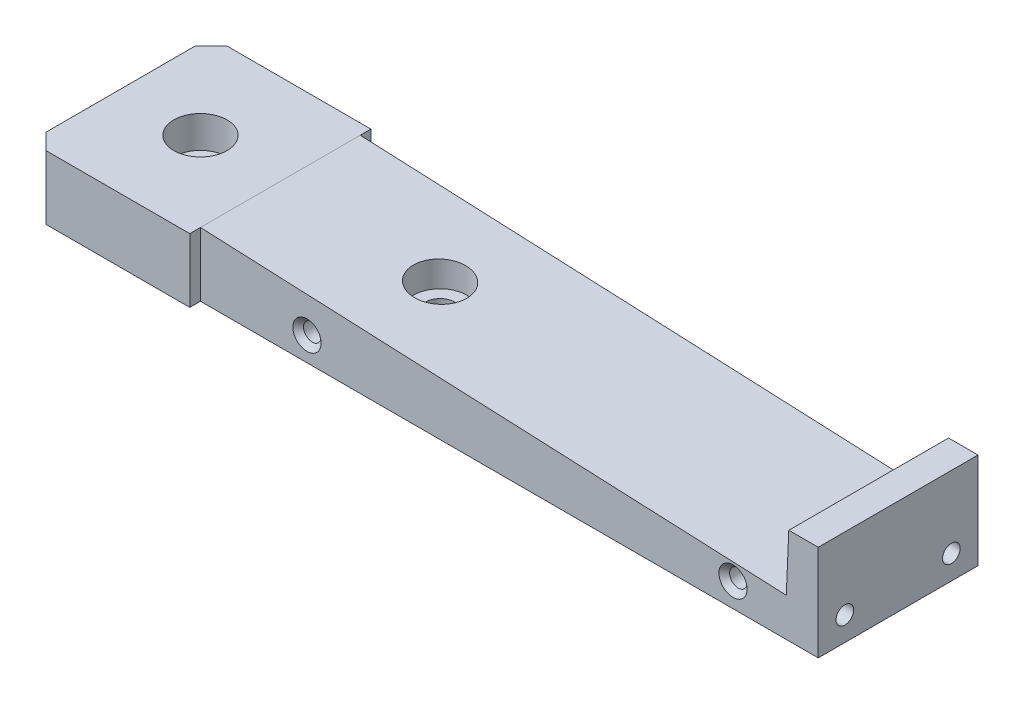
from build123d import *

# Parameters (mm, degrees)
SKETCH1_W                                            = 146
SKETCH1_H                                            = 34
BOSS_EXTRUDE1_DEPTH                                  = 6
HOLE_SIZE_PER_SOCKET_HEAD_CAP_SCREW_TYPE_D           = 5.5
HOLE_SIZE_PER_SOCKET_HEAD_CAP_SCREW_TYPE_CBORE_D     = 10
HOLE_SIZE_PER_SOCKET_HEAD_CAP_SCREW_TYPE_CBORE_DEPTH = 6
M4_TAPPED_HOLE2_D                                    = 3.3
M4_TAPPED_HOLE2_DEPTH                                = 10.1
M4_TAPPED_HOLE2_TIP                                  = 0.991420021
CHAMFER1_SIZE                                        = 3
SKETCH8_W                                            = 116
SKETCH8_H                                            = 2
CUT_EXTRUDE1_DEPTH                                   = 76.907838857
M4_TAPPED_HOLE3_AT_2_COUNT                           = 2
M4_TAPPED_HOLE3_AT_2_PITCH                           = 80
SKETCH11_W                                           = 6
SKETCH11_H                                           = 30
BOSS_EXTRUDE2_DEPTH                                  = 6
CUT_EXTRUDE2_DEPTH                                   = 82.418671077
CUT_EXTRUDE3_DEPTH                                   = 82.418671077
CHAMFER2_SIZE                                        = 1


with BuildPart() as part:
    # Sketch1 → Boss-Extrude1 (new, symmetric)
    with BuildSketch(Plane(origin=(0, 0, 0), x_dir=(1, 0, 0), z_dir=(0, 1, 0))):
        Rectangle(SKETCH1_W, SKETCH1_H)
    extrude(amount=BOSS_EXTRUDE1_DEPTH, both=True)

    # Hole size per socket head cap screw type1 (through all)
    with Locations(Plane(origin=(0, 6, 0), x_dir=(1, 0, 0), z_dir=(0, 1, 0))):
        with Locations((-58, 0), (-13, 0)):
            CounterBoreHole(HOLE_SIZE_PER_SOCKET_HEAD_CAP_SCREW_TYPE_D / 2, HOLE_SIZE_PER_SOCKET_HEAD_CAP_SCREW_TYPE_CBORE_D / 2, HOLE_SIZE_PER_SOCKET_HEAD_CAP_SCREW_TYPE_CBORE_DEPTH)

    # M4 Tapped Hole2
    with Locations(Plane(origin=(73, 0, 0), x_dir=(0, 0, -1), z_dir=(1, 0, 0))):
        with Locations((-10, -1.5), (10, -1.5)):
            Hole(M4_TAPPED_HOLE2_D / 2, depth=M4_TAPPED_HOLE2_DEPTH)
            with Locations((0, 0, -(M4_TAPPED_HOLE2_DEPTH + M4_TAPPED_HOLE2_TIP / 2))):  # 118° drill point
                Cone(0, M4_TAPPED_HOLE2_D / 2, M4_TAPPED_HOLE2_TIP, mode=Mode.SUBTRACT)

    # Chamfer1
    chamfer1_edges = [part.edges().sort_by_distance(p)[0] for p in [
        (-73, 0, 17),
        (-73, 0, -17),
    ]]
    chamfer(chamfer1_edges, length=CHAMFER1_SIZE)

    # Sketch8 → Cut-Extrude1 (cut, through all)
    with BuildSketch(Plane(origin=(0, 6, 0), x_dir=(1, 0, 0), z_dir=(0, 1, 0))):
        with Locations((15, -16)):
            Rectangle(SKETCH8_W, SKETCH8_H)
        with Locations((15, 16)):
            Rectangle(SKETCH8_W, SKETCH8_H)
    extrude(amount=-CUT_EXTRUDE1_DEPTH, mode=Mode.SUBTRACT)

    # Sketch9 → M4 Tapped Hole3 (revolve, cut)
    with BuildSketch(Plane(origin=(-23, -1.5, 15), x_dir=(0, -1, 0), z_dir=(1, 0, 0))):
        Polygon((0, 0), (0, 11.091420021), (1.65, 10.1), (1.65, 0), align=None)
    m4_tapped_hole3 = revolve(axis=Axis((-23, -1.5, 21.35), (0, 0, -1)), mode=Mode.SUBTRACT)

    # M4 Tapped Hole3 at 2: M4 Tapped Hole3 ×2
    with Locations(*[(i * M4_TAPPED_HOLE3_AT_2_PITCH, 0, 0) for i in range(1, M4_TAPPED_HOLE3_AT_2_COUNT)]):
        add(m4_tapped_hole3, mode=Mode.SUBTRACT)

    # Mirror1: M4 Tapped Hole3 across plane
    add(m4_tapped_hole3.mirror(Plane.XY), mode=Mode.SUBTRACT)

    # Mirror1 copy 1 sketch → Mirror1 copy 1 (revolve, cut)
    with BuildSketch(Plane(origin=(57, -1.5, -15), x_dir=(0, -1, 0), z_dir=(1, 0, 0))):
        Polygon((0, 0), (0, -11.091420021), (1.65, -10.1), (1.65, 0), align=None)
    revolve(axis=Axis((57, -1.5, -21.35), (0, 0, -1)), mode=Mode.SUBTRACT)

    # Sketch11 → Boss-Extrude2 (add)
    with BuildSketch(Plane(origin=(0, 6, 0), x_dir=(1, 0, 0), z_dir=(0, 1, 0))):
        with Locations((70, 0)):
            Rectangle(SKETCH11_W, SKETCH11_H)
    extrude(amount=BOSS_EXTRUDE2_DEPTH)

    # Sketch12 → Cut-Extrude2 (cut, through all)
    with BuildSketch(Plane.XY.offset(17)):
        Polygon((67, 6), (-43, 6), (67, 1.19729628), align=None)
    extrude(amount=-CUT_EXTRUDE2_DEPTH, mode=Mode.SUBTRACT)

    # Sketch13 → Cut-Extrude3 (cut, through all)
    with BuildSketch(Plane.XY.offset(17)):
        Polygon((67, 12), (67, 1.19729628), (67.47165623, 12), align=None)
    extrude(amount=-CUT_EXTRUDE3_DEPTH, mode=Mode.SUBTRACT)

    # Chamfer2
    chamfer2_edges = [part.edges().sort_by_distance(p)[0] for p in [
        (57, 0.15, 15),
        (-23, 0.15, 15),
        (57, 0.15, -15),
        (-23, 0.15, -15),
    ]]
    chamfer(chamfer2_edges, length=CHAMFER2_SIZE)


solid = part.part
